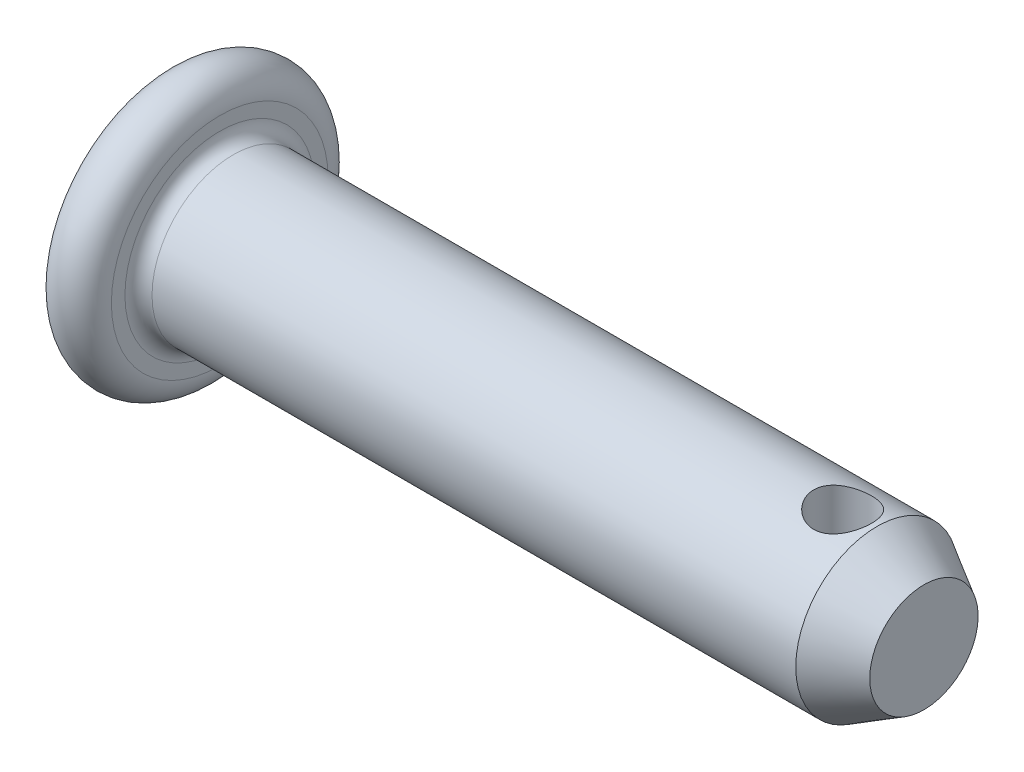
SolidWorks part; units mm, degrees
material "35钢"
ref_plane "前视" through (0, 0, 0) normal (0, 0, 1) x (1, 0, 0)
ref_plane "上视" through (0, 0, 0) normal (0, 1, 0) x (1, 0, 0)
ref_plane "右视" through (0, 0, 0) normal (1, 0, 0) x (0, 0, -1)
sketch "尺寸草图" plane through (0, 0, 0) normal (0, 0, 1) x (1, 0, 0)
  line L0 (0, 10) -> (0, 0)
  line L1 (0, 0) -> (26, 0)
  line L2 (26, 0) -> (29, 0) construction
  point P3 (0, 6)
  point P5 (2, 0)
  point P6 (0.5, 0)
  point P7 (25, 0)
  point P8 (3, 0)
  point P9 (0, 2.14)
sketch "草图1" plane through (0, 0, 0) normal (0, 0, 1) x (1, 0, 0)
  line L0 (0, 0) -> (10.7677, 0) construction
  line L1 (0, 0) -> (28, 0)
  line L2 (0, 0) -> (0, 4)
  line L4 (2, 4) -> (2, 3)
  line L5 (2, 3) -> (28, 3)
  line L6 (28, 3) -> (28, 0)
  arc A0 (0, 4) -> (2, 4) centre (1, 4) cw
revolve "基体-旋转" add sketch "草图1" angle 360 about L0
fillet "圆角1" radius 0.5 1 edges at (2, 0, 3)
chamfer "倒角1" distance 1 angle 60 1 edges at (28, 0, 3)
sketch "草图2" plane through (0, 0, 0) normal (0, 1, 0) x (1, 0, 0)
  line L0 (2, -3.5) -> (2, 3.5) construction
  circle A0 centre (25, 0) radius 1.07
extrude "切除-拉伸1" cut sketch "草图2" against normal mid plane 1000
equation "\"D4@草图1\" = \"K@尺寸草图\""
equation "\"D2@草图1\" = \"dk@尺寸草图\""
equation "\"D1@草图1\" = \"l@尺寸草图\""
equation "\"D3@草图1\" = \"d@尺寸草图\""
equation "\"D1@圆角1\" = \"r@尺寸草图\""
equation "\"D1@倒角1\" = \"c@尺寸草图\""
equation "\"D2@草图2\" = \"d1@尺寸草图\""
equation "\"lh@尺寸草图\" = \"l@尺寸草图\"-\"l-lh@尺寸草图\""
equation "\"D1@草图2\" = \"lh@尺寸草图\""
